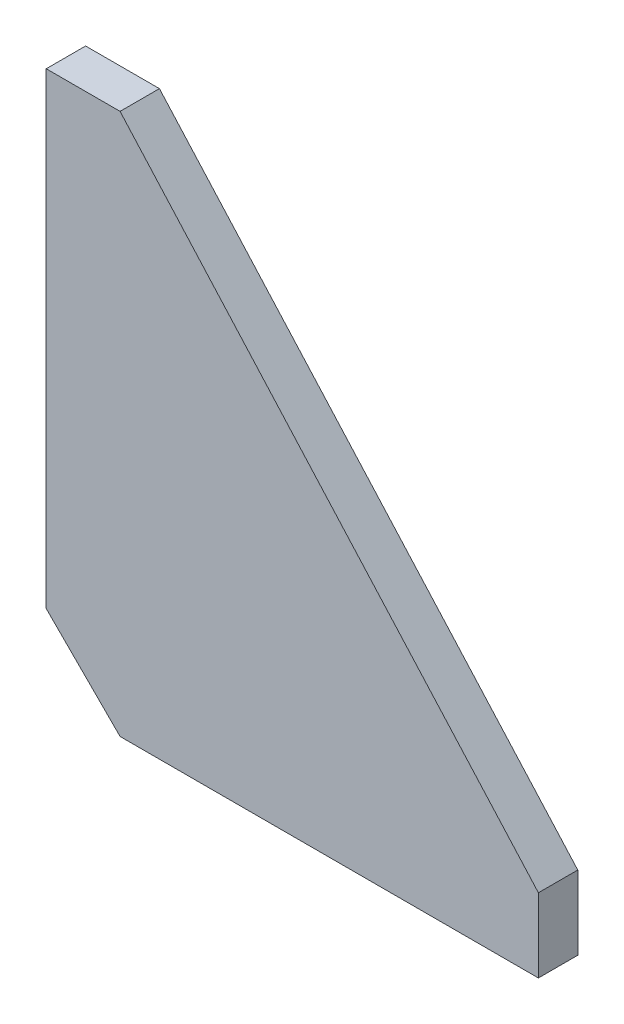
SolidWorks part; units mm, degrees
material "普通碳钢"
ref_plane "前视基准面" through (0, 0, 0) normal (0, 0, 1) x (1, 0, 0)
ref_plane "上视基准面" through (0, 0, 0) normal (0, 1, 0) x (1, 0, 0)
ref_plane "右视基准面" through (0, 0, 0) normal (1, 0, 0) x (0, 0, -1)
sketch "草图1" plane through (0, 0, 0) normal (0, 0, 1) x (1, 0, 0)
  line L0 (0, 0) -> (100, 0)
  line L1 (100, 0) -> (100, 15)
  line L2 (100, 15) -> (15, 110)
  line L3 (15, 110) -> (0, 110)
  line L4 (0, 110) -> (0, 0)
  dimension "D1" = 15
  dimension "D2" = 15
  dimension "D3" = 100
  dimension "D4" = 110
extrude "凸台-拉伸1" add sketch "草图1" along normal blind 8
chamfer "倒角1" distance 15 angle 45 1 edges at (0, 0, 4)
